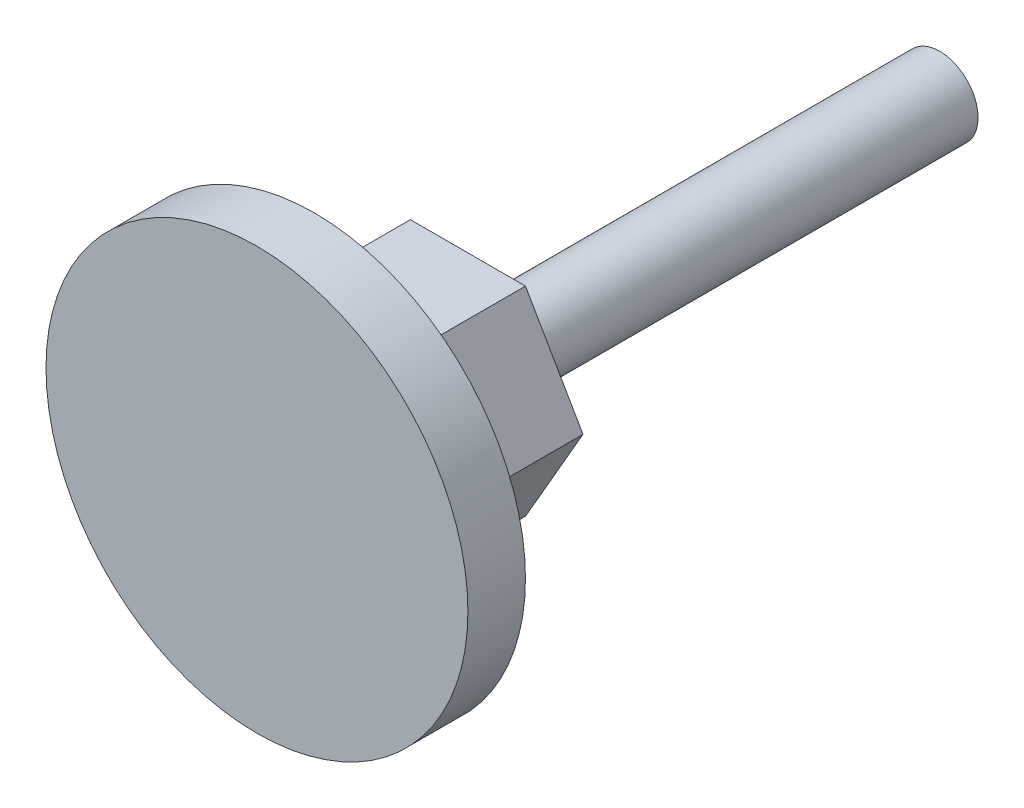
from build123d import *

# Parameters (mm, degrees)
SKETCH_2_R      = 55
EXTRUDE_1_DEPTH = 15
EXTRUDE_2_DEPTH = 25


with BuildPart() as part:
    # 草图1 → 旋转1 (revolve)
    with BuildSketch(Plane(origin=(0, 0, 0), x_dir=(1, 0, 0), z_dir=(0, 1, 0))):
        Polygon((0, 40), (-10, 40), (-10, -108), (-25, -108), (-55, -123), (0, -123), align=None)
    revolve(axis=Axis((0, 0, -40), (0, 0, 1)))

    # 草图2 → 凸台-拉伸1 (add)
    with BuildSketch(Plane.XY.offset(123)):
        Circle(SKETCH_2_R)
    extrude(amount=EXTRUDE_1_DEPTH)

    # 草图3 → 凸台-拉伸2 (add)
    with BuildSketch(Plane(origin=(0, 0, 108), x_dir=(-1, 0, 0), z_dir=(0, 0, -1))):
        Polygon((15, 25.980762114), (-15, 25.980762114), (-30, 0), (-15, -25.980762114), (15, -25.980762114), (30, 0), align=None)
    extrude(amount=EXTRUDE_2_DEPTH)


solid = part.part
